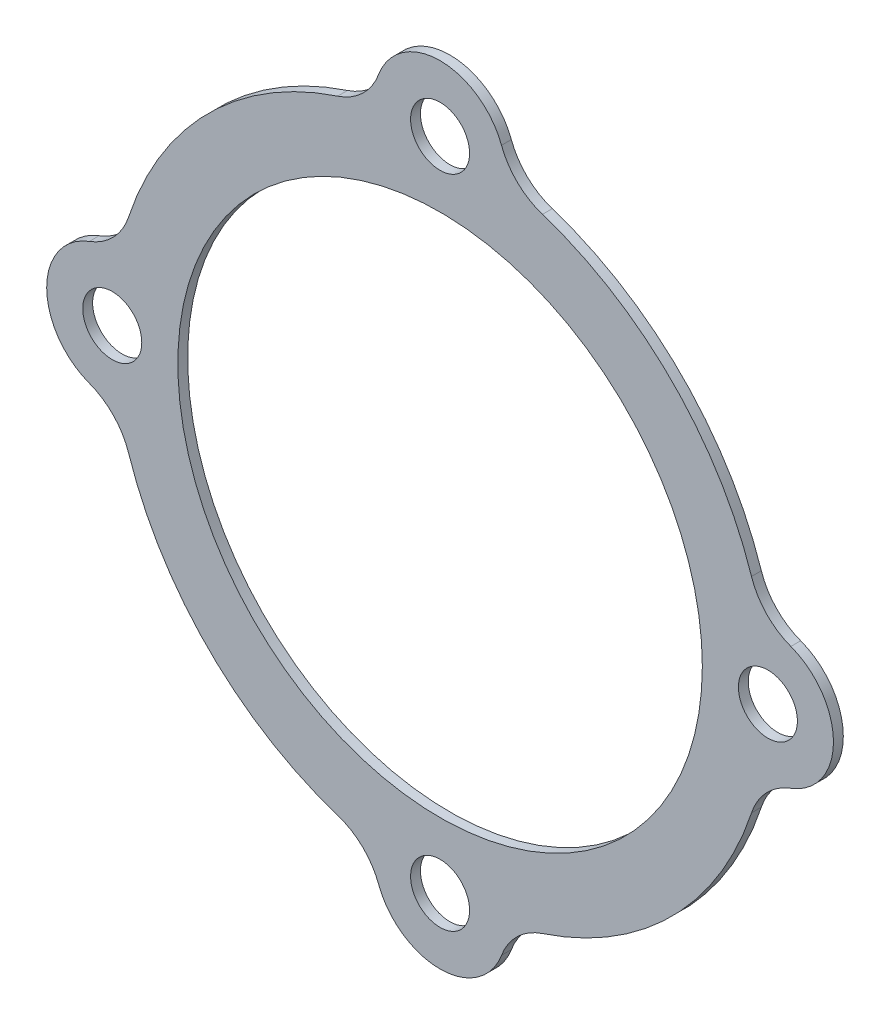
SolidWorks part; units mm, degrees
material "NY250"
ref_plane "前视基准面" through (0, 0, 0) normal (0, 0, 1) x (1, 0, 0)
ref_plane "上视基准面" through (0, 0, 0) normal (0, 1, 0) x (1, 0, 0)
ref_plane "右视基准面" through (0, 0, 0) normal (1, 0, 0) x (0, 0, -1)
sketch "草图1" plane through (0, 0, 0) normal (0, 0, 1) x (1, 0, 0)
  line L0 (0, 0) -> (60, 0) construction
  line L1 (0, 0) -> (-60, 0) construction
  line L2 (0, 0) -> (-60, 0) construction
  line L3 (0, 0) -> (0, 60) construction
  line L4 (0, 0) -> (0, -60) construction
  arc A0 (15.6125, -47.5) -> (47.5, -15.6125) centre (0, 0) ccw
  circle A1 centre (0, 0) radius 40
  circle A2 centre (0, 50) radius 4.5
  circle A3 centre (-50, 0) radius 4.5
  circle A4 centre (0, -50) radius 4.5
  circle A5 centre (50, 0) radius 4.5
  arc A6 (9.3675, 53.5) -> (-9.3675, 53.5) centre (0, 50) ccw
  arc A7 (53.5, -9.3675) -> (53.5, 9.3675) centre (50, 0) ccw
  arc A8 (-53.5, 9.3675) -> (-53.5, -9.3675) centre (-50, 0) ccw
  arc A9 (-9.3675, -53.5) -> (9.3675, -53.5) centre (0, -50) ccw
  arc A10 (-47.5, -15.6125) -> (-15.6125, -47.5) centre (0, 0) ccw
  arc A11 (-15.6125, 47.5) -> (-47.5, 15.6125) centre (0, 0) ccw
  arc A12 (47.5, 15.6125) -> (15.6125, 47.5) centre (0, 0) ccw
  arc A13 (-15.6125, 47.5) -> (-9.3675, 53.5) centre (-18.735, 57) ccw
  arc A14 (15.6125, 47.5) -> (9.3675, 53.5) centre (18.735, 57) cw
  arc A15 (53.5, 9.3675) -> (47.5, 15.6125) centre (57, 18.735) cw
  arc A16 (47.5, -15.6125) -> (53.5, -9.3675) centre (57, -18.735) cw
  arc A17 (9.3675, -53.5) -> (15.6125, -47.5) centre (18.735, -57) cw
  arc A18 (-15.6125, -47.5) -> (-9.3675, -53.5) centre (-18.735, -57) cw
  arc A19 (-53.5, -9.3675) -> (-47.5, -15.6125) centre (-57, -18.735) cw
  arc A20 (-47.5, 15.6125) -> (-53.5, 9.3675) centre (-57, 18.735) cw
  point P26 (-9.9499, 49)
  point P31 (49, 9.9499)
  dimension "D1" = 100
  dimension "D2" = 80
  dimension "D3" = 9
  dimension "D4" = 9
  dimension "D5" = 9
  dimension "D6" = 9
  dimension "D7" = 20
  dimension "D8" = 20
  dimension "D9" = 20
  dimension "D10" = 20
  dimension "D11" = 10
  dimension "D12" = 50
  dimension "D13" = 50
  dimension "D14" = 50
  dimension "D15" = 50
extrude "凸台-拉伸1" add sketch "草图1" along normal blind 1.5
